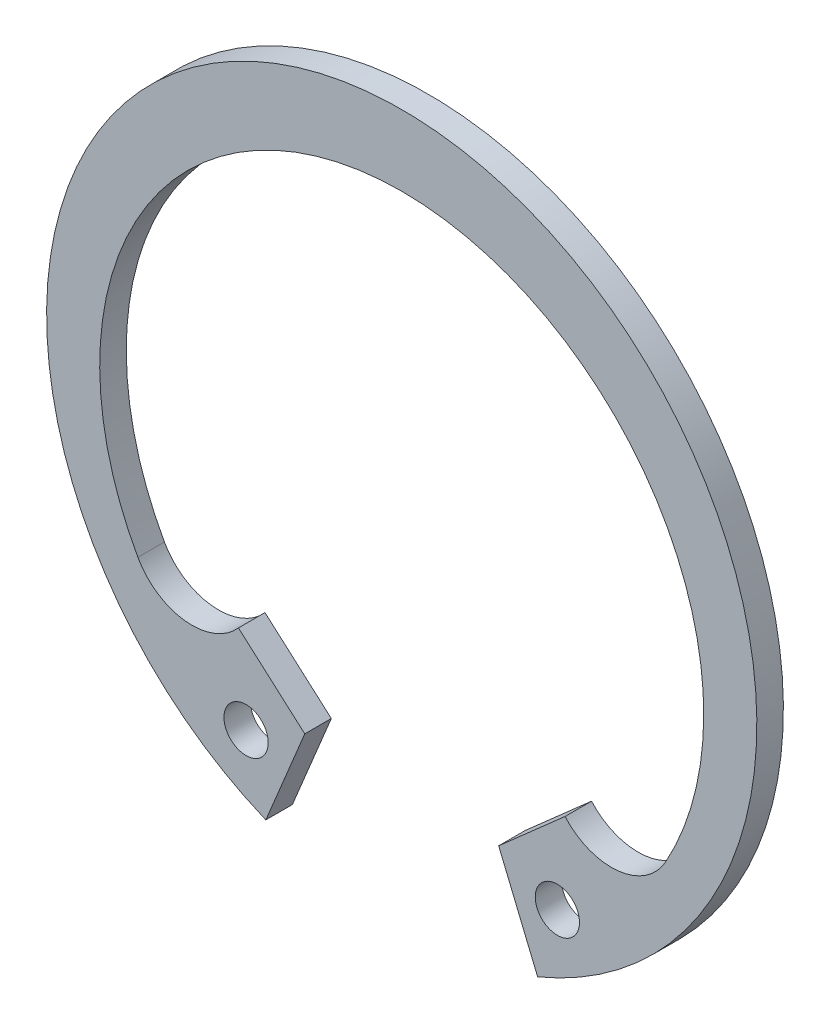
SolidWorks part; units mm, degrees
ref_plane "前视" through (0, 0, 0) normal (0, 0, 1) x (1, 0, 0)
ref_plane "上视" through (0, 0, 0) normal (0, 1, 0) x (1, 0, 0)
ref_plane "右视" through (0, 0, 0) normal (1, 0, 0) x (0, 0, -1)
sketch "草图1" plane through (0, 0, 0) normal (0, 0, 1) x (1, 0, 0)
  line L0 (0, -11.8766) -> (0, 11.8063) construction
  line L1 (0, 0) -> (-4.6199, -11.1535) construction
  line L2 (-7.3805, -7.9313) -> (-4.3817, -10.5784)
  line L3 (-4.3817, -10.5784) -> (-6.1421, -14.8283)
  line L4 (4.3817, -10.5784) -> (6.1421, -14.8283)
  line L5 (7.3805, -7.9313) -> (4.3817, -10.5784)
  arc A0 (6.1421, -14.8283) -> (-6.1421, -14.8283) centre (0, 0) ccw
  arc A1 (11.9259, -7.4404) -> (-11.9259, -7.4404) centre (0, -0.8) ccw
  circle A2 centre (-7.0344, -11.7562) radius 1
  arc A3 (-11.9259, -7.4404) -> (-7.3805, -7.9313) centre (-9.4796, -6.0782) ccw
  circle A4 centre (7.0344, -11.7562) radius 1
  arc A5 (11.9259, -7.4404) -> (7.3805, -7.9313) centre (9.4796, -6.0782) cw
sketch "尺寸草图" plane through (0, 0, 0) normal (0, 0, 1) x (1, 0, 0)
  line L0 (-16.05, 0) -> (16.05, 0) construction
  line L1 (0, 0) -> (29.4981, -33.9833) construction
  circle A2 centre (0, 0) radius 16.05
  point P9 (11.25, 0)
  point P10 (12.05, 0)
  point P11 (-10.9, 0)
  point P12 (-7.7, 0)
  point P13 (4.6, 0)
  point P14 (-11.7, 0)
  point P15 (-15.7, 0)
  point P16 (-13.7, 0)
  point P18 (0.7866, -0.9062)
extrude "基体-拉伸" add sketch "草图1" along normal blind 1.2
equation "\"D1@草图1\" = \"DD@尺寸草图\""
equation "\"D2@草图1\" = \"d@尺寸草图\""
equation "\"D5@草图1\" = \"R2@尺寸草图\""
equation "\"D9@草图1\" = \"R@尺寸草图\""
equation "\"D7@草图1\" = \"B@尺寸草图\""
equation "\"D10@草图1\" = \"B1@尺寸草图\""
equation "\"D4@草图1\" = \"d1@尺寸草图\""
equation "\"D6@草图1\" = \"a@尺寸草图\""
equation "\"D8@草图1\" = \"aa@尺寸草图\"/2"
equation "\"D3@草图1\" = \"c@尺寸草图\""
equation "\"D1@基体-拉伸\"=\"s@尺寸草图\"/2"
equation "\"D2@基体-拉伸\" = \"D1@基体-拉伸\""
